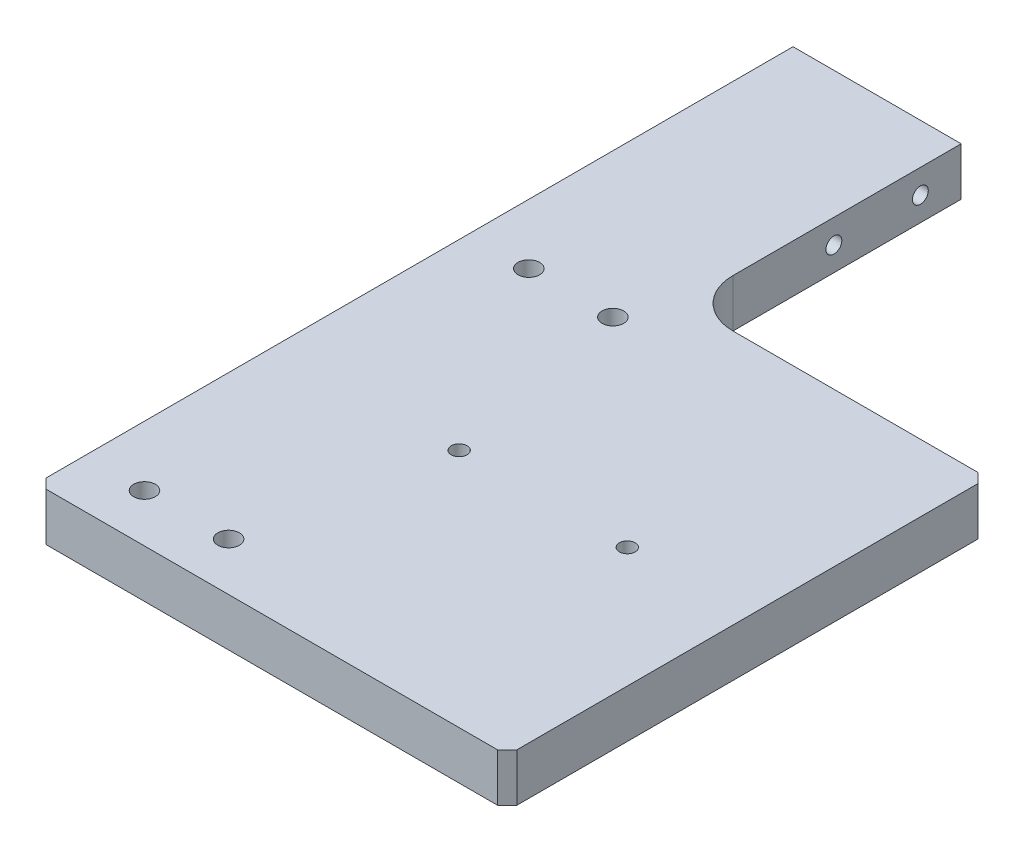
from build123d import *

# Parameters (mm, degrees)
SKETCH_2_W                = 100
SKETCH_2_H                = 10
EXTRUDE_1_DEPTH           = 98
HOLE_WIZARD_1_D           = 4.5
HOLE_WIZARD_1_CBORE_D     = 8
HOLE_WIZARD_1_CBORE_DEPTH = 4.6
CHAMFER_1_SIZE            = 2
HOLE_WIZARD_M4_1_D        = 3.3
SKETCH_9_W                = 35
SKETCH_9_H                = 59.5
EXTRUDE_2_DEPTH           = 10
FILLET_1_R                = 10
HOLE_WIZARD_M4_2_D        = 3.3
HOLE_WIZARD_M4_2_DEPTH    = 11.5
HOLE_WIZARD_M4_2_TIP      = 0.991420021


with BuildPart() as part:
    # 草图2 → 凸台-拉伸1 (new body)
    with BuildSketch(Plane(origin=(0, 0, 0), x_dir=(0, 0, -1), z_dir=(1, 0, 0))):
        Rectangle(SKETCH_2_W, SKETCH_2_H)
    extrude(amount=EXTRUDE_1_DEPTH)

    # 打孔尺寸(%根据)开槽圆柱头螺钉的类型1 (through all)
    with Locations(Plane(origin=(0, -5, 0), x_dir=(-1, 0, 0), z_dir=(0, -1, 0))):
        with Locations((-30, 40), (-30, -40), (-12.5, -40), (-12.5, 40)):
            CounterBoreHole(HOLE_WIZARD_1_D / 2, HOLE_WIZARD_1_CBORE_D / 2, HOLE_WIZARD_1_CBORE_DEPTH)

    # 倒角1
    chamfer_1_edges = [part.edges().sort_by_distance(p)[0] for p in [
        (98, 0, 50),
        (98, 0, -50),
        (0, 0, 50),
        (0, 0, -50),
    ]]
    chamfer(chamfer_1_edges, length=CHAMFER_1_SIZE)

    # M4 螺纹孔1 (through all)
    with Locations(Plane(origin=(0, -5, 0), x_dir=(-1, 0, 0), z_dir=(0, -1, 0))):
        with Locations((-73, 0), (-38, 0)):
            Hole(HOLE_WIZARD_M4_1_D / 2)

    # 草图9 → 凸台-拉伸2 (add)
    with BuildSketch(Plane.XZ.offset(5)):
        with Locations((17.5, -77.75)):
            Rectangle(SKETCH_9_W, SKETCH_9_H)
    extrude(amount=-EXTRUDE_2_DEPTH)

    # 圆角1
    fillet_1_edges = [part.edges().sort_by_distance(p)[0] for p in [
        (35, 0, -50),
    ]]
    fillet(fillet_1_edges, radius=FILLET_1_R)

    # M4 螺纹孔2
    with Locations(Plane(origin=(35, 0, 0), x_dir=(0, 0, -1), z_dir=(1, 0, 0))):
        with Locations((99, 0), (81, 0)):
            Hole(HOLE_WIZARD_M4_2_D / 2, depth=HOLE_WIZARD_M4_2_DEPTH)
            with Locations((0, 0, -(HOLE_WIZARD_M4_2_DEPTH + HOLE_WIZARD_M4_2_TIP / 2))):  # 118° drill point
                Cone(0, HOLE_WIZARD_M4_2_D / 2, HOLE_WIZARD_M4_2_TIP, mode=Mode.SUBTRACT)


solid = part.part
